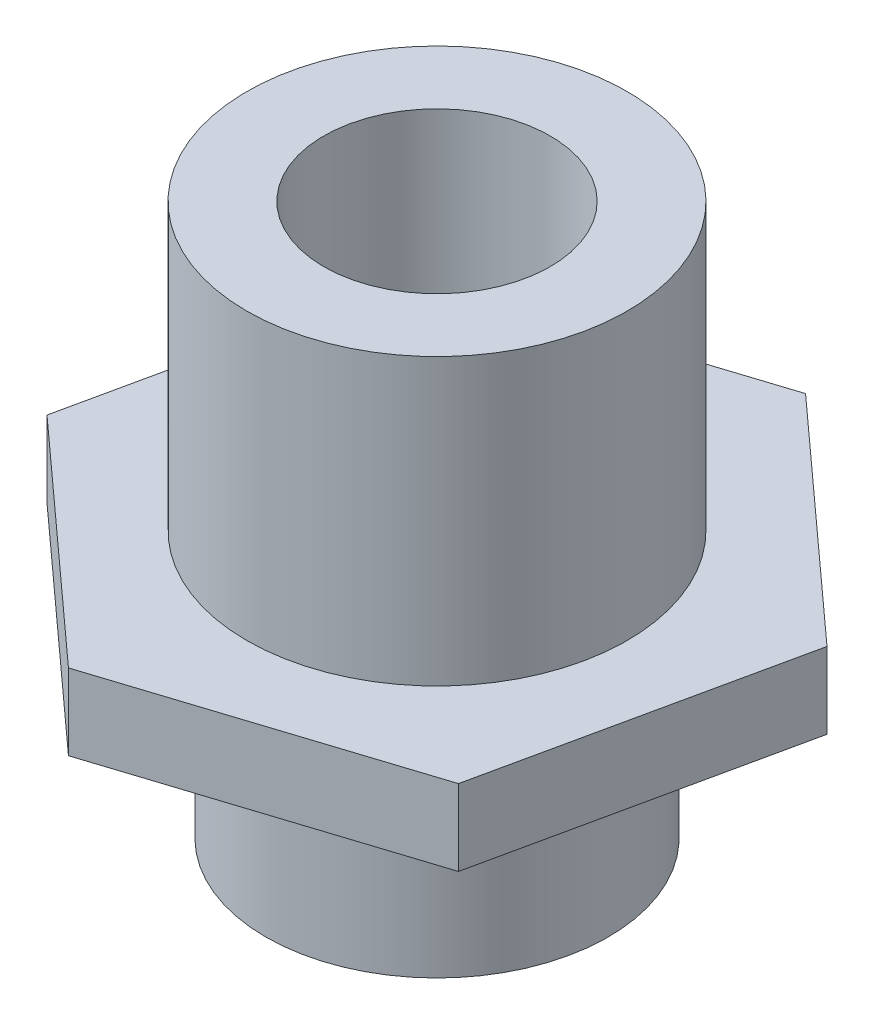
SolidWorks part; units mm, degrees
ref_plane "Front Plane" through (0, 0, 0) normal (0, 0, 1) x (1, 0, 0)
ref_plane "Top Plane" through (0, 0, 0) normal (0, 1, 0) x (1, 0, 0)
ref_plane "Right Plane" through (0, 0, 0) normal (1, 0, 0) x (0, 0, -1)
sketch "Sketch1" plane through (0, 0, 0) normal (0, 1, 0) x (1, 0, 0)
  circle A0 centre (0, 0) radius 9
  circle A1 centre (0, 0) radius 6
  dimension "D1" = 18
  dimension "D2" = 3
extrude "Boss-Extrude1" add sketch "Sketch1" along normal blind 10
sketch "Sketch2" plane through (0, 10, 0) normal (0, 1, 0) x (1, 0, 0)
  line L1 (-12.0764, 10.9484) -> (-15.5197, -4.9843)
  line L2 (-15.5197, -4.9843) -> (-3.4434, -15.9326)
  line L3 (-3.4434, -15.9326) -> (12.0764, -10.9484)
  line L4 (12.0764, -10.9484) -> (15.5197, 4.9843)
  line L5 (15.5197, 4.9843) -> (3.4434, 15.9326)
  line L6 (3.4434, 15.9326) -> (-12.0764, 10.9484)
  circle A0 centre (0, 0) radius 14.1166 construction
  circle A1 centre (0, 0) radius 5.9554
extrude "Boss-Extrude2" add sketch "Sketch2" along normal blind 4 separate body
sketch "Sketch3" plane through (0, 14, 0) normal (0, 1, 0) x (1, 0, 0)
  circle A0 centre (0, 0) radius 10
  circle A1 centre (0, 0) radius 5.9554
extrude "Boss-Extrude3" add sketch "Sketch3" along normal blind 15
